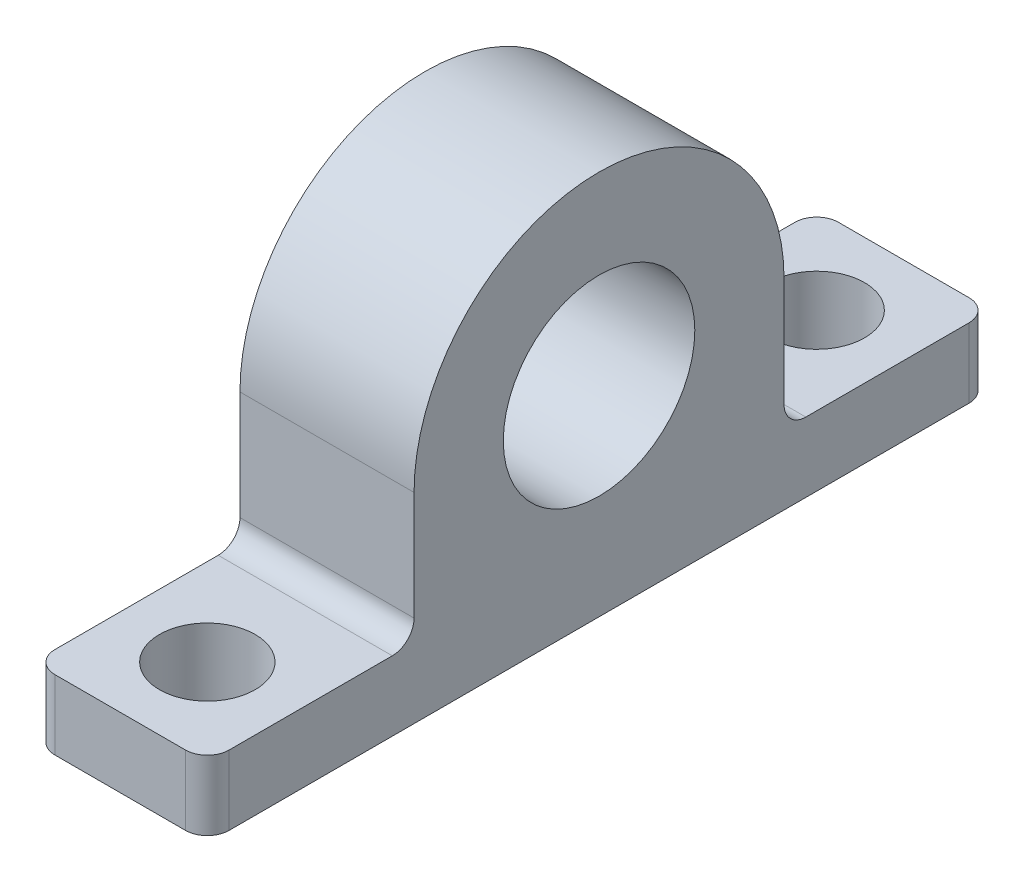
from build123d import *

# Parameters (mm, degrees)
SKETCH1_W           = 40
SKETCH1_H           = 180
SKETCH1_R           = 11
BOSS_EXTRUDE1_DEPTH = 16
SKETCH2_R           = 22
BOSS_EXTRUDE2_DEPTH = 20
FILLET1_R           = 5


with BuildPart() as part:
    # Sketch1 → Boss-Extrude1 (new body)
    with BuildSketch(Plane(origin=(0, 0, 0), x_dir=(1, 0, 0), z_dir=(0, 1, 0))):
        Rectangle(SKETCH1_W, SKETCH1_H)
        with Locations(Location((0, 70, 0), (0, 0, 270))):
            Circle(SKETCH1_R, mode=Mode.SUBTRACT)
        with Locations(Location((0, -70, 0), (0, 0, 90))):
            Circle(SKETCH1_R, mode=Mode.SUBTRACT)
    extrude(amount=BOSS_EXTRUDE1_DEPTH)

    # Sketch2 → Boss-Extrude2 (add, symmetric)
    with BuildSketch(Plane(origin=(0, 0, 0), x_dir=(0, 0, -1), z_dir=(1, 0, 0))):
        with BuildLine():
            Line((-42.5, 46), (-42.5, 16))
            Line((-42.5, 16), (42.5, 16))
            Line((42.5, 16), (42.5, 46))
            ThreePointArc((42.5, 46), (0, 88.5), (-42.5, 46))
        make_face()
        with Locations((0, 46)):
            Circle(SKETCH2_R, mode=Mode.SUBTRACT)
    extrude(amount=BOSS_EXTRUDE2_DEPTH, both=True)

    # Fillet1
    fillet1_edges = [part.edges().sort_by_distance(p)[0] for p in [
        (0, 16, 42.5),
        (20, 8, 90),
        (-20, 8, 90),
        (20, 8, -90),
        (-20, 8, -90),
        (0, 16, -42.5),
    ]]
    fillet(fillet1_edges, radius=FILLET1_R)


solid = part.part
